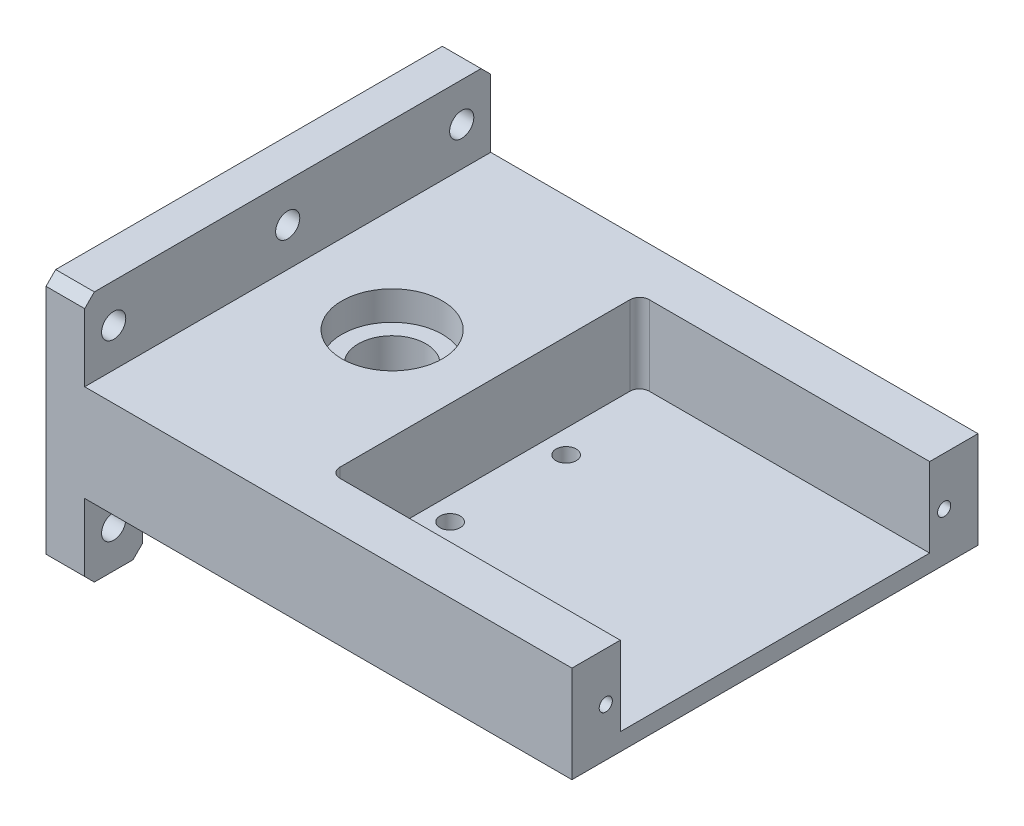
SolidWorks part; units mm, degrees
ref_plane "前视基准面" through (0, 0, 0) normal (0, 0, 1) x (1, 0, 0)
ref_plane "上视基准面" through (0, 0, 0) normal (0, 1, 0) x (1, 0, 0)
ref_plane "右视基准面" through (0, 0, 0) normal (1, 0, 0) x (0, 0, -1)
sketch "草图1" plane through (0, 0, 0) normal (1, 0, 0) x (0, 0, -1)
  line L1 (-105, 65) -> (105, 65)
  line L2 (-105, 65) -> (-105, -65)
  line L3 (-105, -65) -> (105, -65)
  line L4 (105, 65) -> (105, -65)
  line L5 (-105, 65) -> (105, -65) construction
  line L6 (-105, -65) -> (105, 65) construction
  point P0 (0, 0)
  dimension "D1" = 210
  dimension "D2" = 130
extrude "凸台-拉伸1" add sketch "草图1" along normal blind 20
sketch "草图2" plane through (20, 0, 0) normal (1, 0, 0) x (0, 0, -1)
  line L0 (105, -65) -> (105, 65) construction
  line L1 (-105, 25) -> (105, 25)
  line L2 (-105, 25) -> (-105, -25)
  line L3 (-105, -25) -> (105, -25)
  line L4 (105, 25) -> (105, -25)
  line L5 (-105, 25) -> (105, -25) construction
  line L6 (-105, -25) -> (105, 25) construction
  point P0 (0, 0)
  dimension "D1" = 50
extrude "凸台-拉伸2" add sketch "草图2" along normal blind 252
sketch "草图3" plane through (0, 25, 0) normal (0, 1, 0) x (1, 0, 0)
  line L0 (0, 0) -> (156.756, 0) construction
  line L1 (0, 105) -> (0, -105) construction
  circle A0 centre (74, 0) radius 26
  dimension "D1" = 52
  dimension "D2" = 74
extrude "切除-拉伸1" cut sketch "草图3" against normal blind 15
sketch "草图4" plane through (0, 10, 0) normal (0, 1, 0) x (1, 0, 0)
  circle A0 centre (74, 0) radius 17.5
  dimension "D1" = 35
extrude "切除-拉伸2" cut sketch "草图4" against normal through all
sketch "草图5" plane through (272, 0, 0) normal (1, 0, 0) x (0, 0, -1)
  line L0 (105, 25) -> (-105, 25) construction
  line L1 (-80, 25) -> (80, 25)
  line L2 (-80, 25) -> (-80, -16)
  line L3 (-80, -16) -> (80, -16)
  line L4 (80, 25) -> (80, -16)
  line L5 (0, 0) -> (0, 70.5694) construction
  dimension "D1" = 160
  dimension "D2" = 41
extrude "切除-拉伸3" cut sketch "草图5" against normal blind 150
hole_wizard "M8 螺纹孔1" positions "草图6" profile "草图7" tap size "M8" standard "GB"
sketch "草图6" plane through (272, 0, 0) normal (1, 0, 0) x (0, 0, -1)
  line L0 (0, 0) -> (-161.4093, 0) construction
  line L2 (0, 0) -> (0, 91.5456) construction
  point P0 (-87.5, 0)
  point P2 (87.5, 0)
  dimension "D1" = 175
sketch "草图7" plane through (272, 0, 87.5) normal (0, 1, 0) x (0, 0, -1)
  line L0 (0, 0) -> (0, 21.7929)
  line L1 (0, 21.7929) -> (3.4, 19.75)
  line L2 (3.4, 19.75) -> (3.4, 0)
  line L5 (3.4, 0) -> (0, 0)
  line L10 (0, 21.7929) -> (-3.4, 19.75) construction
  line L11 (0, -6.35) -> (0, 107.95) construction
  dimension "螺纹孔钻头直径" = 6.8
  dimension "螺纹孔钻头深度" = 19.75
  dimension "导头角度" = 118
cosmetic thread "孔螺蚊线1" parameters "D1"=16, "D2"=8
cosmetic thread "孔螺蚊线2" parameters "D1"=16, "D2"=8
hole_wizard "Ø10.5 (10.5) 直径孔1" positions "草图8" profile "草图9" hole size "Ø10.5" standard "ISO" end condition through all
sketch "草图8" plane through (0, -25, 0) normal (0, -1, 0) x (-1, 0, 0)
  line L0 (0, 0) -> (-351.2352, 0) construction
  line L2 (-272, -105) -> (-272, 105) construction
  point P0 (-134, 30)
  point P2 (-134, -30)
  dimension "D1" = 138
  dimension "D2" = 60
sketch "草图9" plane through (134, -25, -30) normal (1, 0, 0) x (0, 0, -1)
  line L0 (0, 0) -> (0, 90)
  line L1 (0, 90) -> (5.25, 90)
  line L2 (5.25, 90) -> (5.25, 0)
  line L5 (5.25, 0) -> (0, 0)
  line L11 (0, -6.35) -> (0, 107.95) construction
  dimension "通孔孔直径" = 10.5
  dimension "通孔孔深度" = 90
sketch "草图10" plane through (20, 0, 0) normal (1, 0, 0) x (0, 0, -1)
  line L0 (-105, -65) -> (105, -65) construction
  line L1 (-75, -65) -> (75, -65)
  line L2 (-75, -65) -> (-75, -25)
  line L3 (-75, -25) -> (75, -25)
  line L4 (75, -65) -> (75, -25)
  line L5 (-105, -25) -> (105, -25) construction
  line L6 (0, 0) -> (0, -94.3415) construction
  dimension "D1" = 150
extrude "切除-拉伸4" cut sketch "草图10" against normal through all
hole_wizard "Ø12.5 (12.5) 直径孔1" positions "草图11" profile "草图12" hole size "Ø12.5" standard "ISO" end condition through all
sketch "草图11" plane through (20, 0, 0) normal (1, 0, 0) x (0, 0, -1)
  line L0 (0, 0) -> (0, -62.3809) construction
  line L2 (0, 0) -> (144.5929, 0) construction
  point P0 (-90, 45)
  point P2 (0, 45)
  point P4 (90, 45)
  point P6 (-90, -45)
  point P8 (90, -45)
  dimension "D1" = 90
  dimension "D2" = 180
sketch "草图12" plane through (20, 45, 90) normal (0, 1, 0) x (0, 0, -1)
  line L0 (0, 0) -> (0, 20)
  line L1 (0, 20) -> (6.25, 20)
  line L2 (6.25, 20) -> (6.25, 0)
  line L5 (6.25, 0) -> (0, 0)
  line L11 (0, -6.35) -> (0, 107.95) construction
  dimension "通孔孔直径" = 12.5
  dimension "通孔孔深度" = 20
chamfer "倒角1" distance 5 angle 45 6 edges at (10, 65, -105) (10, -65, -75) (10, -65, -105) (10, -65, 75) (10, -65, 105) (10, 65, 105)
fillet "圆角1" radius 5 2 edges at (122, 4.5, 80) (122, 4.5, -80)
